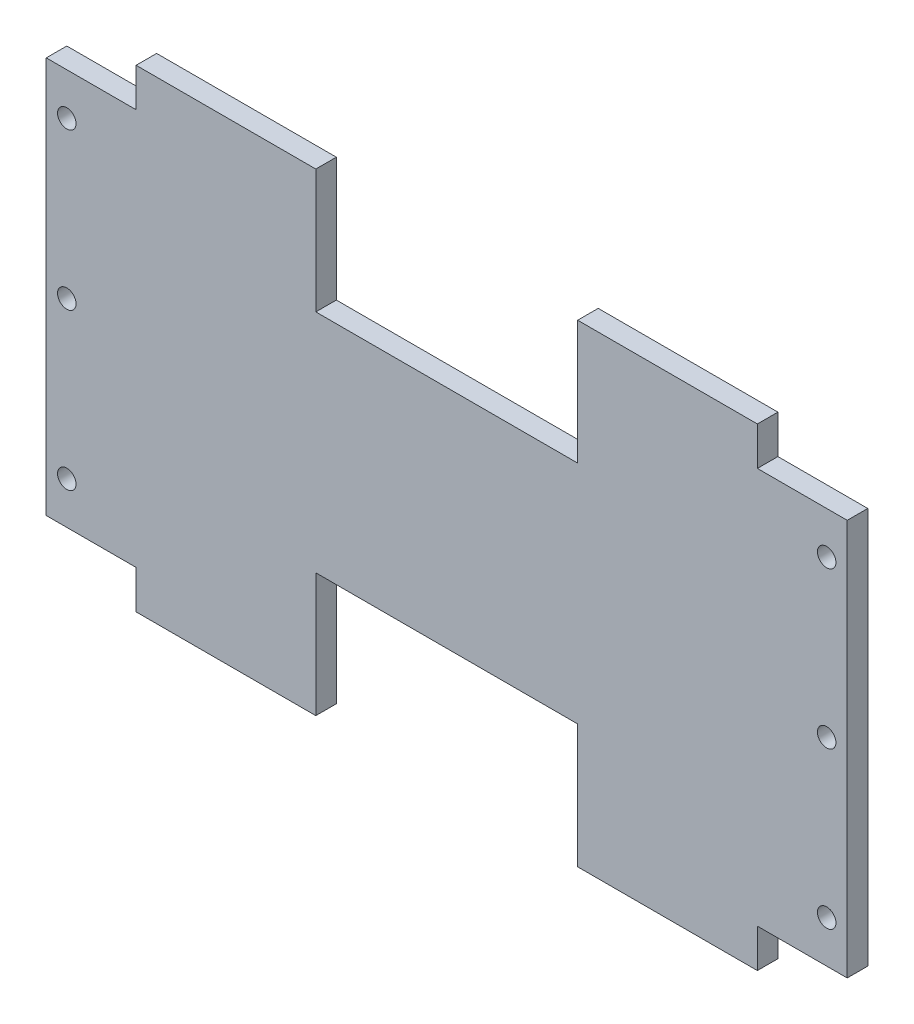
from build123d import *

# Parameters (mm, degrees)
SKETCH1_R           = 18
BOSS_EXTRUDE1_DEPTH = 40


with BuildPart() as part:
    # Sketch1 → Boss-Extrude1 (new body)
    with BuildSketch(Plane.XY):
        Polygon((255, 0), (-255, 0), (-255, -241), (-605, -241), (-605, -166), (-780, -166), (-780, 606), (-605, 606), (-605, 681), (-255, 681), (-255, 440), (255, 440), (255, 681), (605, 681), (605, 606), (780, 606), (780, -166), (605, -166), (605, -241), (255, -241), align=None)
        with Locations((-740, 524)):
            Circle(SKETCH1_R, mode=Mode.SUBTRACT)
        with Locations((-740, 220)):
            Circle(SKETCH1_R, mode=Mode.SUBTRACT)
        with Locations((-740, -84)):
            Circle(SKETCH1_R, mode=Mode.SUBTRACT)
        with Locations(Location((740, 220, 0), (0, 0, 180))):
            Circle(SKETCH1_R, mode=Mode.SUBTRACT)
        with Locations(Location((740, 524, 0), (0, 0, 180))):
            Circle(SKETCH1_R, mode=Mode.SUBTRACT)
        with Locations(Location((740, -84, 0), (0, 0, 180))):
            Circle(SKETCH1_R, mode=Mode.SUBTRACT)
    extrude(amount=BOSS_EXTRUDE1_DEPTH)


solid = part.part
